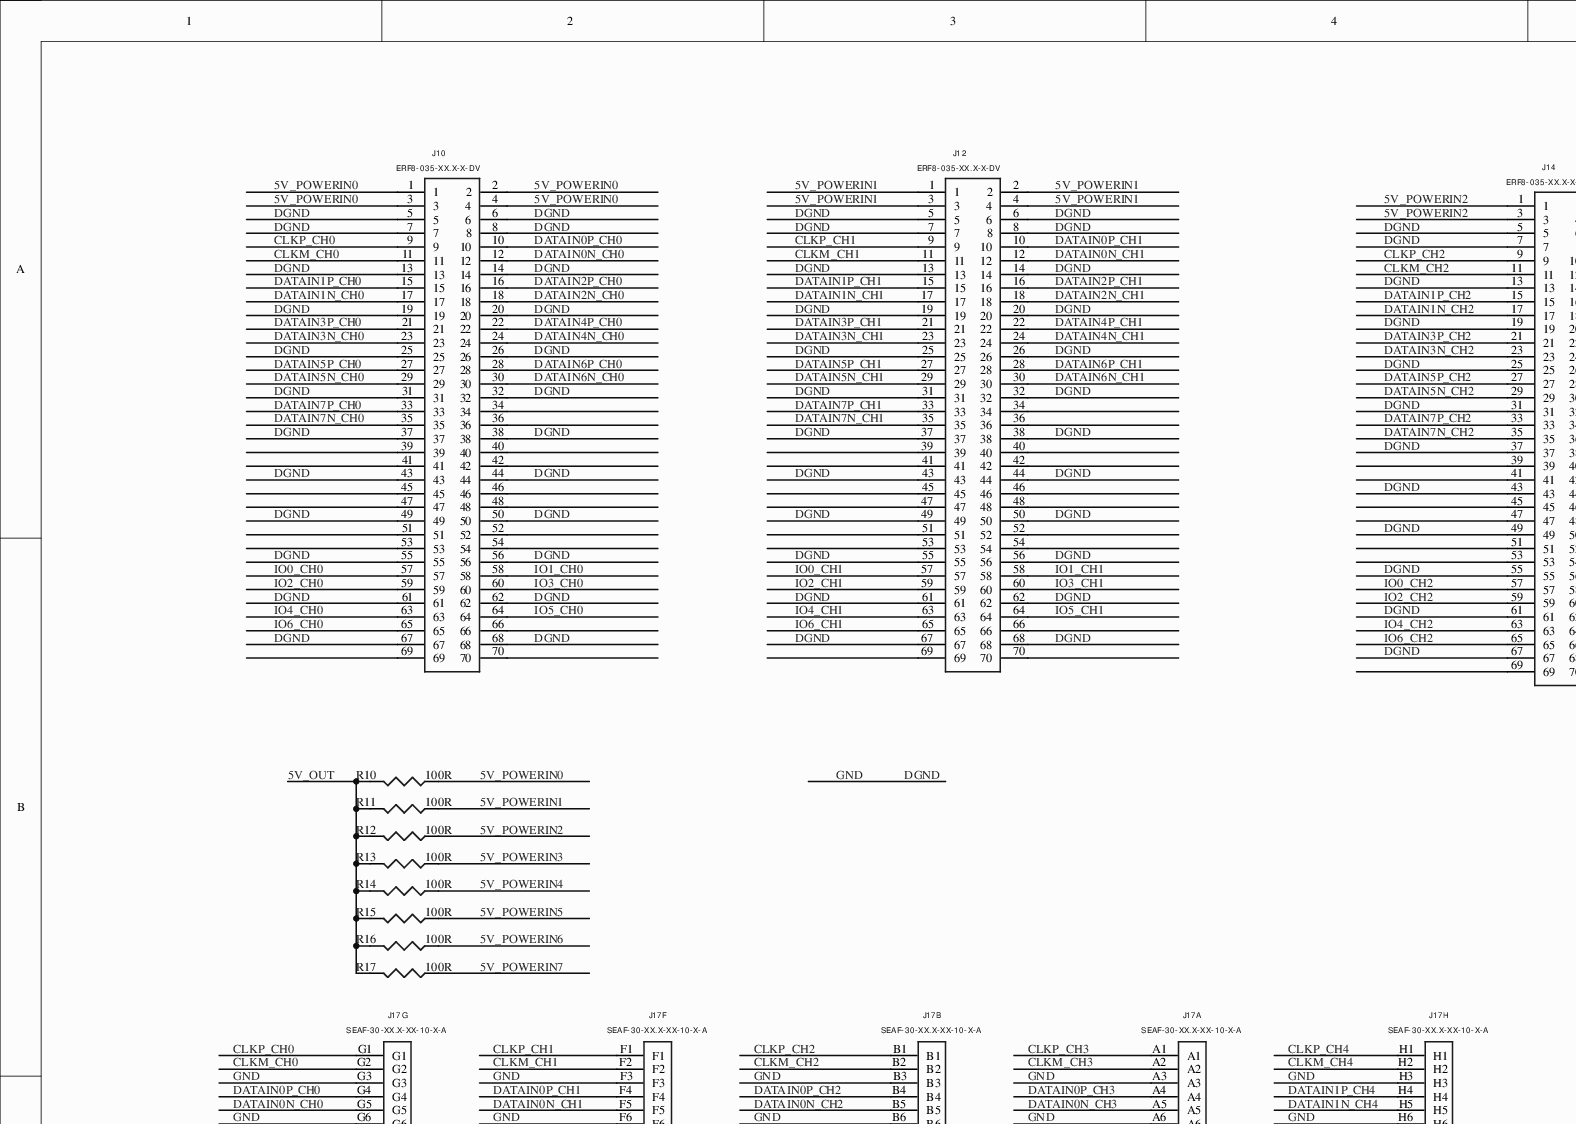
[diagram p0: MISC86329.SchDoc, top left]
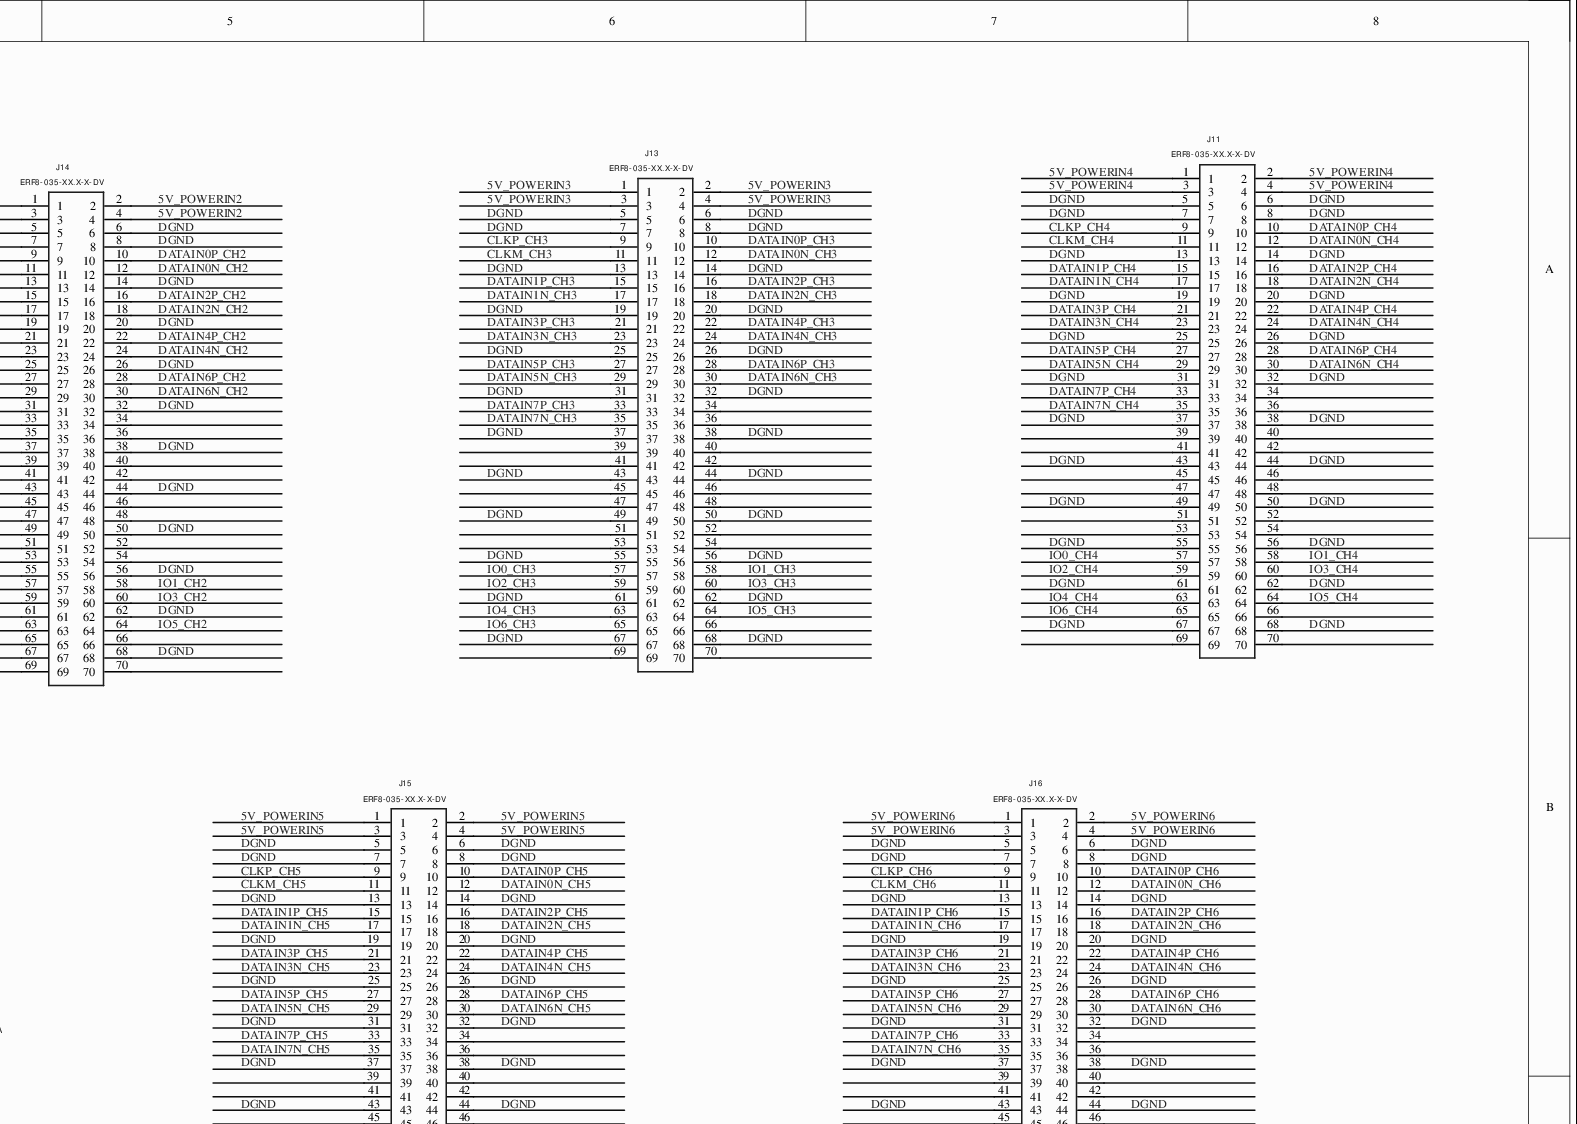
[diagram p1: MISC86329.SchDoc, top right]
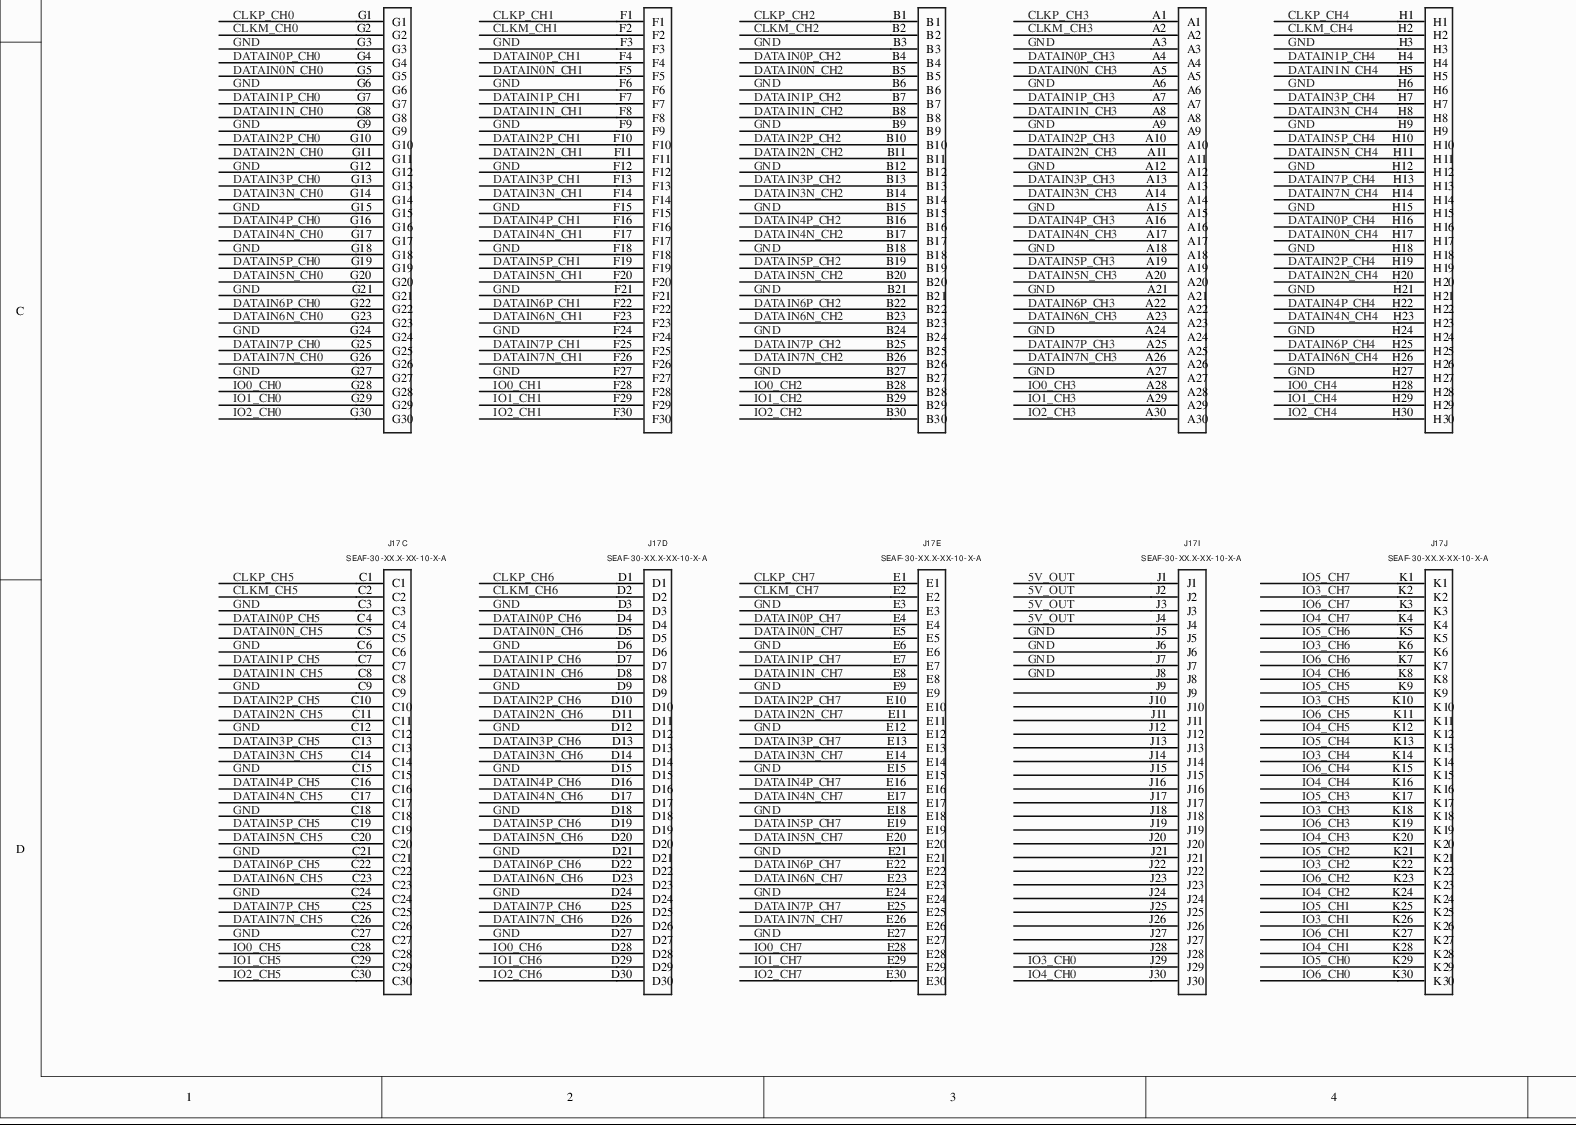
[diagram p2: MISC86329.SchDoc, bottom left]
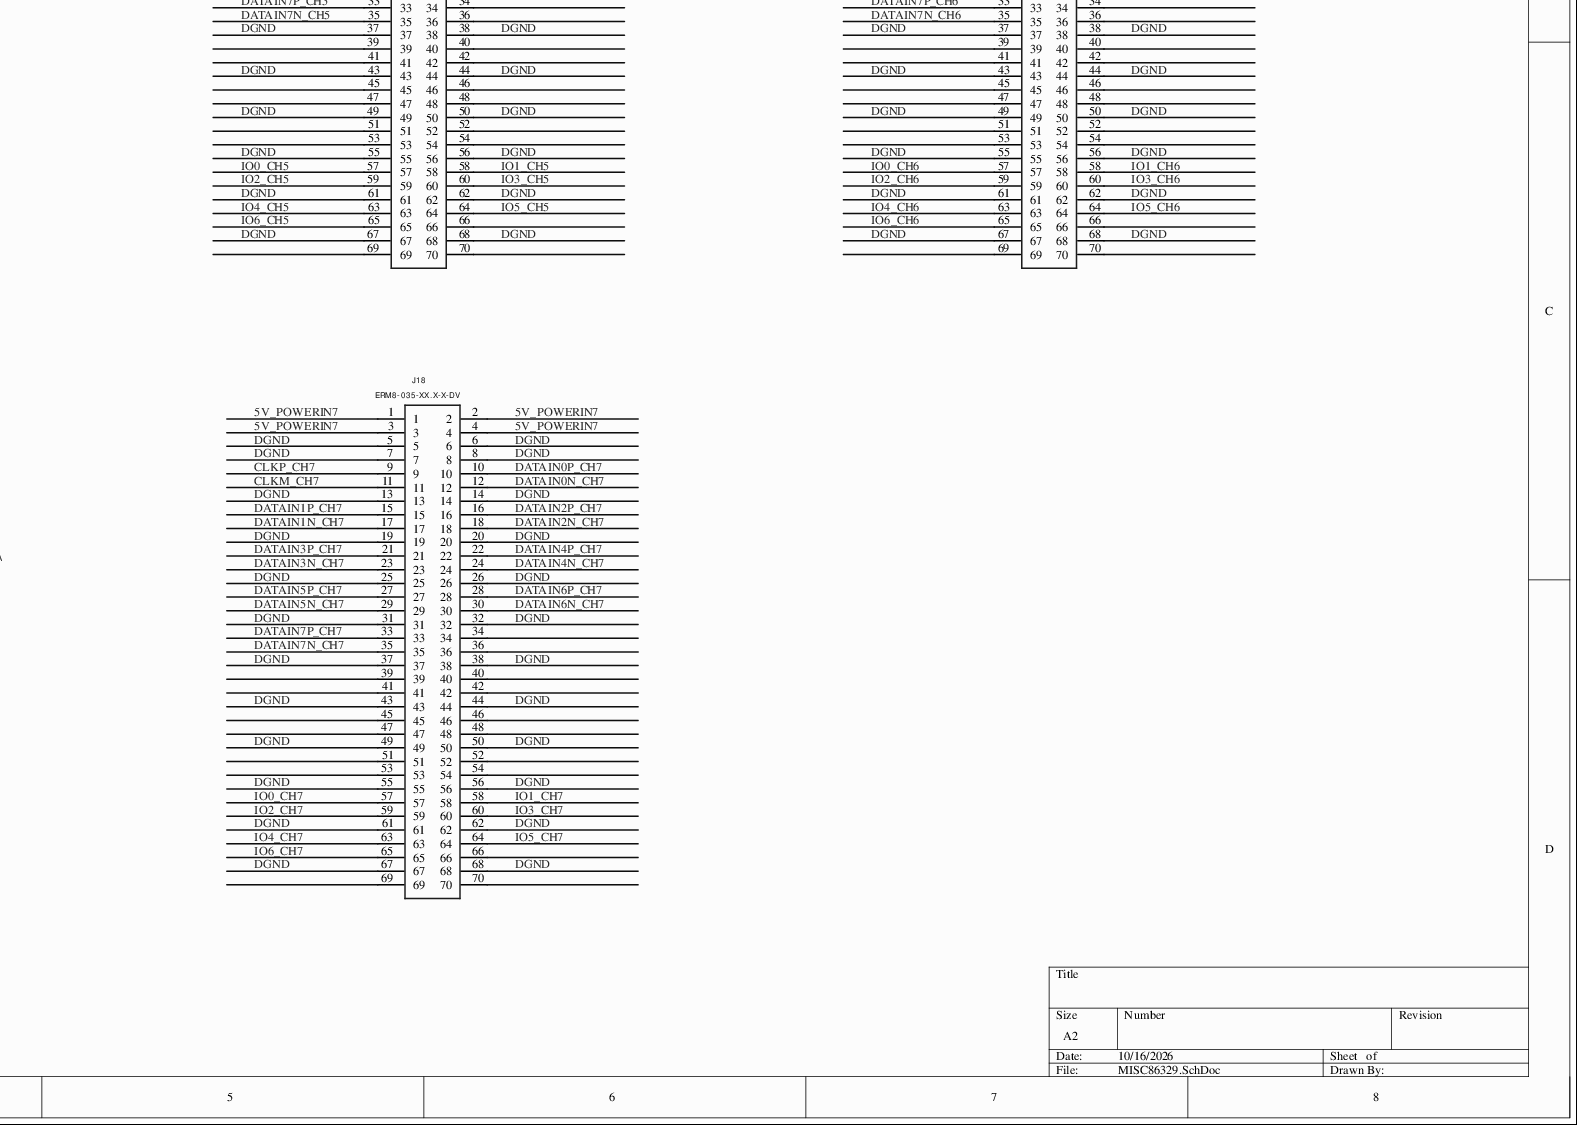
[diagram p3: MISC86329.SchDoc, bottom right]
# Altium project MISC86329.PrjPCB
1 sheet, 17 parts. Net scope: global (net labels, ports and power ports of the same name join across sheets).
Board file: MISC86329.PcbDoc

## Sheet MISC86329.SchDoc
size A2

### Parts
J10  ERF8-035-XX.X-X-DV  [ERF8-035-XX.X-X-DV]
J11  ERF8-035-XX.X-X-DV  [ERF8-035-XX.X-X-DV]
J12  ERF8-035-XX.X-X-DV  [ERF8-035-XX.X-X-DV]
J13  ERF8-035-XX.X-X-DV  [ERF8-035-XX.X-X-DV]
J14  ERF8-035-XX.X-X-DV  [ERF8-035-XX.X-X-DV]
J15  ERF8-035-XX.X-X-DV  [ERF8-035-XX.X-X-DV]
J16  ERF8-035-XX.X-X-DV  [ERF8-035-XX.X-X-DV]
J17  SEAF-30-XX.X-XX-10-X-A  [SEAF-30-XX.X-XX-10-X-A]  (parts A,B,C,D,E,F,G,H,I,J of 10)
J18  ERM8-035-XX.X-X-DV  [ERF8-035-XX.X-X-DV]
R10  100R  [R1210]
R11  100R  [R1210]
R12  100R  [R1210]
R13  100R  [R1210]
R14  100R  [R1210]
R15  100R  [R1210]
R16  100R  [R1210]
R17  100R  [R1210]

### Nets
5V_OUT: J17.J1 J17.J2 J17.J3 J17.J4 R10.2 R11.2 R12.2 R13.2 R14.2 R15.2 R16.2 R17.2
5V_POWERIN0: J10.1 J10.2 J10.3 J10.4 R10.1
5V_POWERIN1: J12.1 J12.2 J12.3 J12.4 R11.1
5V_POWERIN2: J14.1 J14.2 J14.3 J14.4 R12.1
5V_POWERIN3: J13.1 J13.2 J13.3 J13.4 R13.1
5V_POWERIN4: J11.1 J11.2 J11.3 J11.4 R14.1
5V_POWERIN5: J15.1 J15.2 J15.3 J15.4 R15.1
5V_POWERIN6: J16.1 J16.2 J16.3 J16.4 R16.1
5V_POWERIN7: J18.1 J18.2 J18.3 J18.4 R17.1
CLKM_CH0: J10.11 J17.G2
CLKM_CH1: J12.11 J17.F2
CLKM_CH2: J14.11 J17.B2
CLKM_CH3: J13.11 J17.A2
CLKM_CH4: J11.11 J17.H2
CLKM_CH5: J15.11 J17.C2
CLKM_CH6: J16.11 J17.D2
CLKM_CH7: J17.E2 J18.11
CLKP_CH0: J10.9 J17.G1
CLKP_CH1: J12.9 J17.F1
CLKP_CH2: J14.9 J17.B1
CLKP_CH3: J13.9 J17.A1
CLKP_CH4: J11.9 J17.H1
CLKP_CH5: J15.9 J17.C1
CLKP_CH6: J16.9 J17.D1
CLKP_CH7: J17.E1 J18.9
DATAIN0N_CH0: J10.12 J17.G5
DATAIN0N_CH1: J12.12 J17.F5
DATAIN0N_CH2: J14.12 J17.B5
DATAIN0N_CH3: J13.12 J17.A5
DATAIN0N_CH4: J11.12 J17.H17
DATAIN0N_CH5: J15.12 J17.C5
DATAIN0N_CH6: J16.12 J17.D5
DATAIN0N_CH7: J17.E5 J18.12
DATAIN0P_CH0: J10.10 J17.G4
DATAIN0P_CH1: J12.10 J17.F4
DATAIN0P_CH2: J14.10 J17.B4
DATAIN0P_CH3: J13.10 J17.A4
DATAIN0P_CH4: J11.10 J17.H16
DATAIN0P_CH5: J15.10 J17.C4
DATAIN0P_CH6: J16.10 J17.D4
DATAIN0P_CH7: J17.E4 J18.10
DATAIN1N_CH0: J10.17 J17.G8
DATAIN1N_CH1: J12.17 J17.F8
DATAIN1N_CH2: J14.17 J17.B8
DATAIN1N_CH3: J13.17 J17.A8
DATAIN1N_CH4: J11.17 J17.H5
DATAIN1N_CH5: J15.17 J17.C8
DATAIN1N_CH6: J16.17 J17.D8
DATAIN1N_CH7: J17.E8 J18.17
DATAIN1P_CH0: J10.15 J17.G7
DATAIN1P_CH1: J12.15 J17.F7
DATAIN1P_CH2: J14.15 J17.B7
DATAIN1P_CH3: J13.15 J17.A7
DATAIN1P_CH4: J11.15 J17.H4
DATAIN1P_CH5: J15.15 J17.C7
DATAIN1P_CH6: J16.15 J17.D7
DATAIN1P_CH7: J17.E7 J18.15
DATAIN2N_CH0: J10.18 J17.G11
DATAIN2N_CH1: J12.18 J17.F11
DATAIN2N_CH2: J14.18 J17.B11
DATAIN2N_CH3: J13.18 J17.A11
DATAIN2N_CH4: J11.18 J17.H20
DATAIN2N_CH5: J15.18 J17.C11
DATAIN2N_CH6: J16.18 J17.D11
DATAIN2N_CH7: J17.E11 J18.18
DATAIN2P_CH0: J10.16 J17.G10
DATAIN2P_CH1: J12.16 J17.F10
DATAIN2P_CH2: J14.16 J17.B10
DATAIN2P_CH3: J13.16 J17.A10
DATAIN2P_CH4: J11.16 J17.H19
DATAIN2P_CH5: J15.16 J17.C10
DATAIN2P_CH6: J16.16 J17.D10
DATAIN2P_CH7: J17.E10 J18.16
DATAIN3N_CH0: J10.23 J17.G14
DATAIN3N_CH1: J12.23 J17.F14
DATAIN3N_CH2: J14.23 J17.B14
DATAIN3N_CH3: J13.23 J17.A14
DATAIN3N_CH4: J11.23 J17.H8
DATAIN3N_CH5: J15.23 J17.C14
DATAIN3N_CH6: J16.23 J17.D14
DATAIN3N_CH7: J17.E14 J18.23
DATAIN3P_CH0: J10.21 J17.G13
DATAIN3P_CH1: J12.21 J17.F13
DATAIN3P_CH2: J14.21 J17.B13
DATAIN3P_CH3: J13.21 J17.A13
DATAIN3P_CH4: J11.21 J17.H7
DATAIN3P_CH5: J15.21 J17.C13
DATAIN3P_CH6: J16.21 J17.D13
DATAIN3P_CH7: J17.E13 J18.21
DATAIN4N_CH0: J10.24 J17.G17
DATAIN4N_CH1: J12.24 J17.F17
DATAIN4N_CH2: J14.24 J17.B17
DATAIN4N_CH3: J13.24 J17.A17
DATAIN4N_CH4: J11.24 J17.H23
DATAIN4N_CH5: J15.24 J17.C17
DATAIN4N_CH6: J16.24 J17.D17
DATAIN4N_CH7: J17.E17 J18.24
DATAIN4P_CH0: J10.22 J17.G16
DATAIN4P_CH1: J12.22 J17.F16
DATAIN4P_CH2: J14.22 J17.B16
DATAIN4P_CH3: J13.22 J17.A16
DATAIN4P_CH4: J11.22 J17.H22
DATAIN4P_CH5: J15.22 J17.C16
DATAIN4P_CH6: J16.22 J17.D16
DATAIN4P_CH7: J17.E16 J18.22
DATAIN5N_CH0: J10.29 J17.G20
DATAIN5N_CH1: J12.29 J17.F20
DATAIN5N_CH2: J14.29 J17.B20
DATAIN5N_CH3: J13.29 J17.A20
DATAIN5N_CH4: J11.29 J17.H11
DATAIN5N_CH5: J15.29 J17.C20
DATAIN5N_CH6: J16.29 J17.D20
DATAIN5N_CH7: J17.E20 J18.29
DATAIN5P_CH0: J10.27 J17.G19
DATAIN5P_CH1: J12.27 J17.F19
DATAIN5P_CH2: J14.27 J17.B19
DATAIN5P_CH3: J13.27 J17.A19
DATAIN5P_CH4: J11.27 J17.H10
DATAIN5P_CH5: J15.27 J17.C19
DATAIN5P_CH6: J16.27 J17.D19
DATAIN5P_CH7: J17.E19 J18.27
DATAIN6N_CH0: J10.30 J17.G23
DATAIN6N_CH1: J12.30 J17.F23
DATAIN6N_CH2: J14.30 J17.B23
DATAIN6N_CH3: J13.30 J17.A23
DATAIN6N_CH4: J11.30 J17.H26
DATAIN6N_CH5: J15.30 J17.C23
DATAIN6N_CH6: J16.30 J17.D23
DATAIN6N_CH7: J17.E23 J18.30
DATAIN6P_CH0: J10.28 J17.G22
DATAIN6P_CH1: J12.28 J17.F22
DATAIN6P_CH2: J14.28 J17.B22
DATAIN6P_CH3: J13.28 J17.A22
DATAIN6P_CH4: J11.28 J17.H25
DATAIN6P_CH5: J15.28 J17.C22
DATAIN6P_CH6: J16.28 J17.D22
DATAIN6P_CH7: J17.E22 J18.28
DATAIN7N_CH0: J10.35 J17.G26
DATAIN7N_CH1: J12.35 J17.F26
DATAIN7N_CH2: J14.35 J17.B26
DATAIN7N_CH3: J13.35 J17.A26
DATAIN7N_CH4: J11.35 J17.H14
DATAIN7N_CH5: J15.35 J17.C26
DATAIN7N_CH6: J16.35 J17.D26
DATAIN7N_CH7: J17.E26 J18.35
DATAIN7P_CH0: J10.33 J17.G25
DATAIN7P_CH1: J12.33 J17.F25
DATAIN7P_CH2: J14.33 J17.B25
DATAIN7P_CH3: J13.33 J17.A25
DATAIN7P_CH4: J11.33 J17.H13
DATAIN7P_CH5: J15.33 J17.C25
DATAIN7P_CH6: J16.33 J17.D25
DATAIN7P_CH7: J17.E25 J18.33
DGND: J10.5 J10.6 J10.7 J10.8 J10.13 J10.14 J10.19 J10.20 J10.25 J10.26 J10.31 J10.32 J10.37 J10.38 J10.43 J10.44 J10.49 J10.50 J10.55 J10.56 J10.61 J10.62 J10.67 J10.68 J11.5 J11.6 J11.7 J11.8 J11.13 J11.14 J11.19 J11.20 J11.25 J11.26 J11.31 J11.32 J11.37 J11.38 J11.43 J11.44 J11.49 J11.50 J11.55 J11.56 J11.61 J11.62 J11.67 J11.68 J12.5 J12.6 J12.7 J12.8 J12.13 J12.14 J12.19 J12.20 J12.25 J12.26 J12.31 J12.32 J12.37 J12.38 J12.43 J12.44 J12.49 J12.50 J12.55 J12.56 J12.61 J12.62 J12.67 J12.68 J13.5 J13.6 J13.7 J13.8 J13.13 J13.14 J13.19 J13.20 J13.25 J13.26 J13.31 J13.32 J13.37 J13.38 J13.43 J13.44 J13.49 J13.50 J13.55 J13.56 J13.61 J13.62 J13.67 J13.68 J14.5 J14.6 J14.7 J14.8 J14.13 J14.14 J14.19 J14.20 J14.25 J14.26 J14.31 J14.32 J14.37 J14.38 J14.43 J14.44 J14.49 J14.50 J14.55 J14.56 J14.61 J14.62 J14.67 J14.68 J15.5 J15.6 J15.7 J15.8 J15.13 J15.14 J15.19 J15.20 J15.25 J15.26 J15.31 J15.32 J15.37 J15.38 J15.43 J15.44 J15.49 J15.50 J15.55 J15.56 J15.61 J15.62 J15.67 J15.68 J16.5 J16.6 J16.7 J16.8 J16.13 J16.14 J16.19 J16.20 J16.25 J16.26 J16.31 J16.32 J16.37 J16.38 J16.43 J16.44 J16.49 J16.50 J16.55 J16.56 J16.61 J16.62 J16.67 J16.68 J17.A3 J17.A6 J17.A9 J17.A12 J17.A15 J17.A18 J17.A21 J17.A24 J17.A27 J17.B3 J17.B6 J17.B9 J17.B12 J17.B15 J17.B18 J17.B21 J17.B24 J17.B27 J17.C3 J17.C6 J17.C9 J17.C12 J17.C15 J17.C18 J17.C21 J17.C24 J17.C27 J17.D3 J17.D6 J17.D9 J17.D12 J17.D15 J17.D18 J17.D21 J17.D24 J17.D27 J17.E3 J17.E6 J17.E9 J17.E12 J17.E15 J17.E18 J17.E21 J17.E24 J17.E27 J17.F3 J17.F6 J17.F9 J17.F12 J17.F15 J17.F18 J17.F21 J17.F24 J17.F27 J17.G3 J17.G6 J17.G9 J17.G12 J17.G15 J17.G18 J17.G21 J17.G24 J17.G27 J17.H3 J17.H6 J17.H9 J17.H12 J17.H15 J17.H18 J17.H21 J17.H24 J17.H27 J17.J5 J17.J6 J17.J7 J17.J8 J18.5 J18.6 J18.7 J18.8 J18.13 J18.14 J18.19 J18.20 J18.25 J18.26 J18.31 J18.32 J18.37 J18.38 J18.43 J18.44 J18.49 J18.50 J18.55 J18.56 J18.61 J18.62 J18.67 J18.68  [also labelled GND]
IO0_CH0: J10.57 J17.G28
IO0_CH1: J12.57 J17.F28
IO0_CH2: J14.57 J17.B28
IO0_CH3: J13.57 J17.A28
IO0_CH4: J11.57 J17.H28
IO0_CH5: J15.57 J17.C28
IO0_CH6: J16.57 J17.D28
IO0_CH7: J17.E28 J18.57
IO1_CH0: J10.58 J17.G29
IO1_CH1: J12.58 J17.F29
IO1_CH2: J14.58 J17.B29
IO1_CH3: J13.58 J17.A29
IO1_CH4: J11.58 J17.H29
IO1_CH5: J15.58 J17.C29
IO1_CH6: J16.58 J17.D29
IO1_CH7: J17.E29 J18.58
IO2_CH0: J10.59 J17.G30
IO2_CH1: J12.59 J17.F30
IO2_CH2: J14.59 J17.B30
IO2_CH3: J13.59 J17.A30
IO2_CH4: J11.59 J17.H30
IO2_CH5: J15.59 J17.C30
IO2_CH6: J16.59 J17.D30
IO2_CH7: J17.E30 J18.59
IO3_CH0: J10.60 J17.J29
IO3_CH1: J12.60 J17.K26
IO3_CH2: J14.60 J17.K22
IO3_CH3: J13.60 J17.K18
IO3_CH4: J11.60 J17.K14
IO3_CH5: J15.60 J17.K10
IO3_CH6: J16.60 J17.K6
IO3_CH7: J17.K2 J18.60
IO4_CH0: J10.63 J17.J30
IO4_CH1: J12.63 J17.K28
IO4_CH2: J14.63 J17.K24
IO4_CH3: J13.63 J17.K20
IO4_CH4: J11.63 J17.K16
IO4_CH5: J15.63 J17.K12
IO4_CH6: J16.63 J17.K8
IO4_CH7: J17.K4 J18.63
IO5_CH0: J10.64 J17.K29
IO5_CH1: J12.64 J17.K25
IO5_CH2: J14.64 J17.K21
IO5_CH3: J13.64 J17.K17
IO5_CH4: J11.64 J17.K13
IO5_CH5: J15.64 J17.K9
IO5_CH6: J16.64 J17.K5
IO5_CH7: J17.K1 J18.64
IO6_CH0: J10.65 J17.K30
IO6_CH1: J12.65 J17.K27
IO6_CH2: J14.65 J17.K23
IO6_CH3: J13.65 J17.K19
IO6_CH4: J11.65 J17.K15
IO6_CH5: J15.65 J17.K11
IO6_CH6: J16.65 J17.K7
IO6_CH7: J17.K3 J18.65

Not connected (* = marked no-connect by the designer): J10 34 36 39 40 41 42 45 46 47 48 51 52 53 54 66 69 70; J11 34 36 39 40 41 42 45 46 47 48 51 52 53 54 66 69 70; J12 34 36 39 40 41 42 45 46 47 48 51 52 53 54 66 69 70; J13 34 36 39 40 41 42 45 46 47 48 51 52 53 54 66 69 70; J14 34 36 39 40 41 42 45 46 47 48 51 52 53 54 66 69 70; J15 34 36 39 40 41 42 45 46 47 48 51 52 53 54 66 69 70; J16 34 36 39 40 41 42 45 46 47 48 51 52 53 54 66 69 70; J17 J9* J10* J11* J12* J13* J14* J15* J16* J17* J18* J19* J20* J21* J22* J23* J24* J25* J26* J27* J28*; J18 34 36 39 40 41 42 45 46 47 48 51 52 53 54 66 69 70

### Library data of the parts
J10-J16 = ERF8-035-XX.X-X-DV: 0.8mm Edge Rate Socket Assembly, Double Vertical Row, 30 Positions Per Row.; MANUFACTURER: SAMTEC; PCB DECAL: ERF8-035-XX.X-X-DV; CREATED: January 10, 2017 - PERSON_A
J17 = SEAF-30-XX.X-XX-10-X-A: Socket Array Assembly, Surface Mount, 0.050" Pitch, 300 Pins; MANUFACTURER: SAMTEC; PCB DECAL: SEAF-30-XX.X-XX-10-X-A; CREATED: March 24, 2015 - PERSON_A
J18 = ERM8-035-XX.X-X-DV: 0.8mm Edge Rate Terminal Assembly, Double Vertical Row, 40 Position, 0.8mm Pitch; Factory: SAMTEC; ProductID: ERM8-035-XX.X-X-DV
R10-R17 = Res_4K7_0.05_1608[0603]_FENGHUA: Resistor; Factory: YAGEO; ProductID: RC0603FR-0733KL; Parameter: 1%10W; Sub-Type: 1%